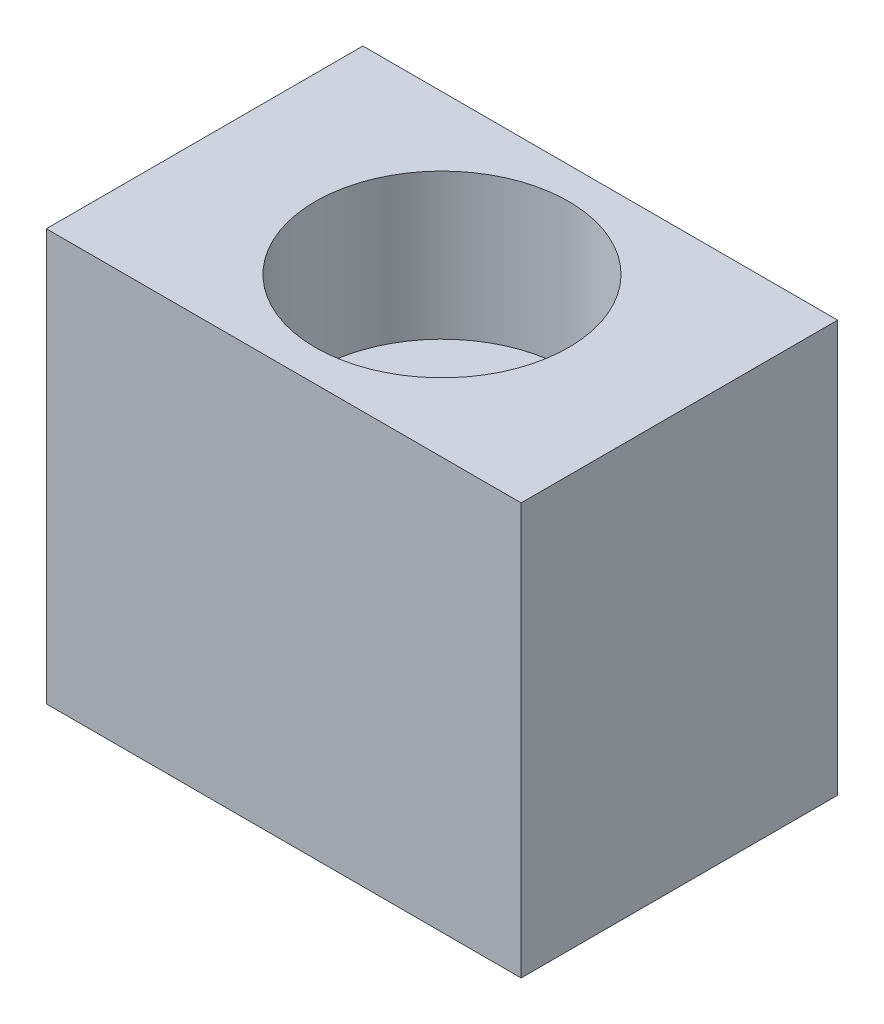
from build123d import *

# Parameters (mm, degrees)
SKETCH_1_W                = 15
SKETCH_1_H                = 10
EXTRUDE_1_DEPTH           = 6.5
HOLE_WIZARD_1_D           = 4.5
HOLE_WIZARD_1_CBORE_D     = 8
HOLE_WIZARD_1_CBORE_DEPTH = 4.6


with BuildPart() as part:
    # 草图1 → 凸台-拉伸1 (new, symmetric)
    with BuildSketch(Plane(origin=(0, 0, 0), x_dir=(1, 0, 0), z_dir=(0, 1, 0))):
        Rectangle(SKETCH_1_W, SKETCH_1_H)
    extrude(amount=EXTRUDE_1_DEPTH, both=True)

    # 打孔尺寸(%根据)内六角圆柱头螺钉的类型1 (through all)
    with Locations(Plane(origin=(0, 6.5, 0), x_dir=(1, 0, 0), z_dir=(0, 1, 0))):
        with Locations((0, 0)):
            CounterBoreHole(HOLE_WIZARD_1_D / 2, HOLE_WIZARD_1_CBORE_D / 2, HOLE_WIZARD_1_CBORE_DEPTH)


solid = part.part
